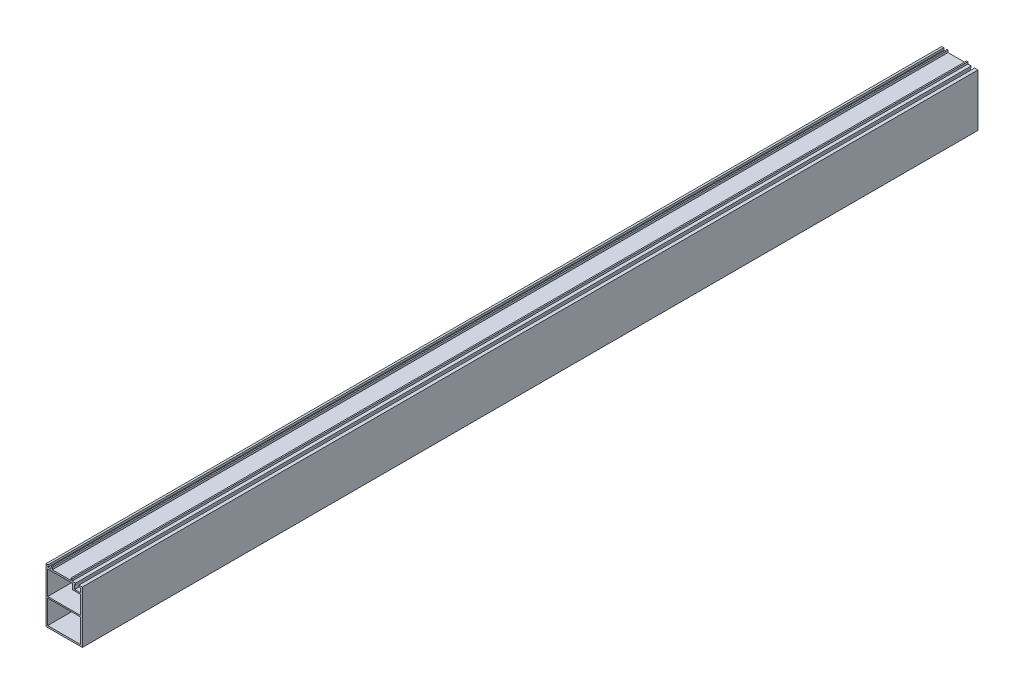
from build123d import *

# Parameters (mm, degrees)
SKETCH1_W           = 39
SKETCH1_H           = 28.2
BOSS_EXTRUDE1_DEPTH = 530


with BuildPart() as part:
    # Sketch1 → Boss-Extrude1 (new, symmetric)
    with BuildSketch(Plane.XY):
        Polygon((21.5, -31), (-21.5, -31), (-21.5, 31), (-21.5, 33.5), (-19, 33.5), (-19, 31), (-15.5, 31), (-15.5, 33.5), (-14, 33.5), (-14, 31), (8, 31), (8, 33.5), (9.5, 33.5), (9.5, 31), (13.5, 31), (13.5, 29), (12.5, 29), (12.5, 24), (19.5, 24), (19.5, 29), (17.5, 29), (17.5, 31), (21.5, 31), align=None)
        Polygon((19.5, 0.8), (-19.5, 0.8), (-19.5, 29), (10.1, 29), (10.1, 22.4), (19.5, 22.4), align=None, mode=Mode.SUBTRACT)
        with Locations((0, -14.9)):
            Rectangle(SKETCH1_W, SKETCH1_H, mode=Mode.SUBTRACT)
    extrude(amount=BOSS_EXTRUDE1_DEPTH, both=True)


solid = part.part
